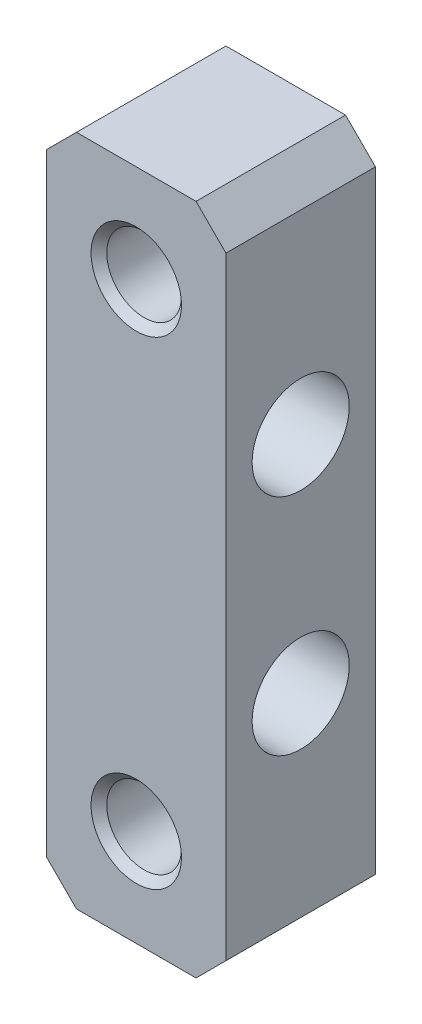
from build123d import *

# Parameters (mm, degrees)
SKETCH_1_W                   = 12
SKETCH_1_H                   = 45
EXTRUDE_1_DEPTH              = 5
HOLE_WIZARD_M6_1_D           = 5
HOLE_WIZARD_M6_1_CSINK_D     = 6.05
HOLE_WIZARD_M6_1_CSINK_ANGLE = 90
CUT_EXTRUDE_1_REACH          = 27.986
SKETCH_3_R                   = 3.25
CHAMFER_1_SIZE               = 2


with BuildPart() as part:
    # 草图1 → 凸台-拉伸1 (new, symmetric)
    with BuildSketch(Plane.XY):
        Rectangle(SKETCH_1_W, SKETCH_1_H)
    extrude(amount=EXTRUDE_1_DEPTH, both=True)

    # M6 螺纹孔1 (through all)
    with Locations(Plane(origin=(0, -16, 5), x_dir=(1, 0, 0), z_dir=(0, 0, 1))):
        with Locations((0, 0)):
            hole_wizard_m6_1 = CounterSinkHole(HOLE_WIZARD_M6_1_D / 2, HOLE_WIZARD_M6_1_CSINK_D / 2, counter_sink_angle=HOLE_WIZARD_M6_1_CSINK_ANGLE)

    # 草图3 → 切除-拉伸1 (cut, up to next)
    with BuildSketch(Plane.ZY.offset(6), mode=Mode.PRIVATE) as cut_extrude_1_sk1:
        with Locations((0, 7.5)):
            Circle(SKETCH_3_R)
    cut_extrude_1_tool1 = extrude(cut_extrude_1_sk1.sketch, amount=-CUT_EXTRUDE_1_REACH, mode=Mode.PRIVATE) & part.part
    # 草图3 → 切除-拉伸1 (cut, up to next)
    with BuildSketch(Plane.ZY.offset(6), mode=Mode.PRIVATE) as cut_extrude_1_sk2:
        with Locations((0, -7.5)):
            Circle(SKETCH_3_R)
    cut_extrude_1_tool2 = extrude(cut_extrude_1_sk2.sketch, amount=-CUT_EXTRUDE_1_REACH, mode=Mode.PRIVATE) & part.part
    add(cut_extrude_1_tool1.solids().sort_by_distance((-6, 7.5, 0))[0], mode=Mode.SUBTRACT)
    add(cut_extrude_1_tool2.solids().sort_by_distance((-6, -7.5, 0))[0], mode=Mode.SUBTRACT)

    # 镜向1: M6 螺纹孔1 across plane
    add(hole_wizard_m6_1.mirror(Plane.ZX), mode=Mode.SUBTRACT)

    # 倒角1
    chamfer_1_edges = [part.edges().sort_by_distance(p)[0] for p in [
        (6, -22.5, 0),
        (-6, -22.5, 0),
        (-6, 22.5, 0),
        (6, 22.5, 0),
    ]]
    chamfer(chamfer_1_edges, length=CHAMFER_1_SIZE)


solid = part.part
